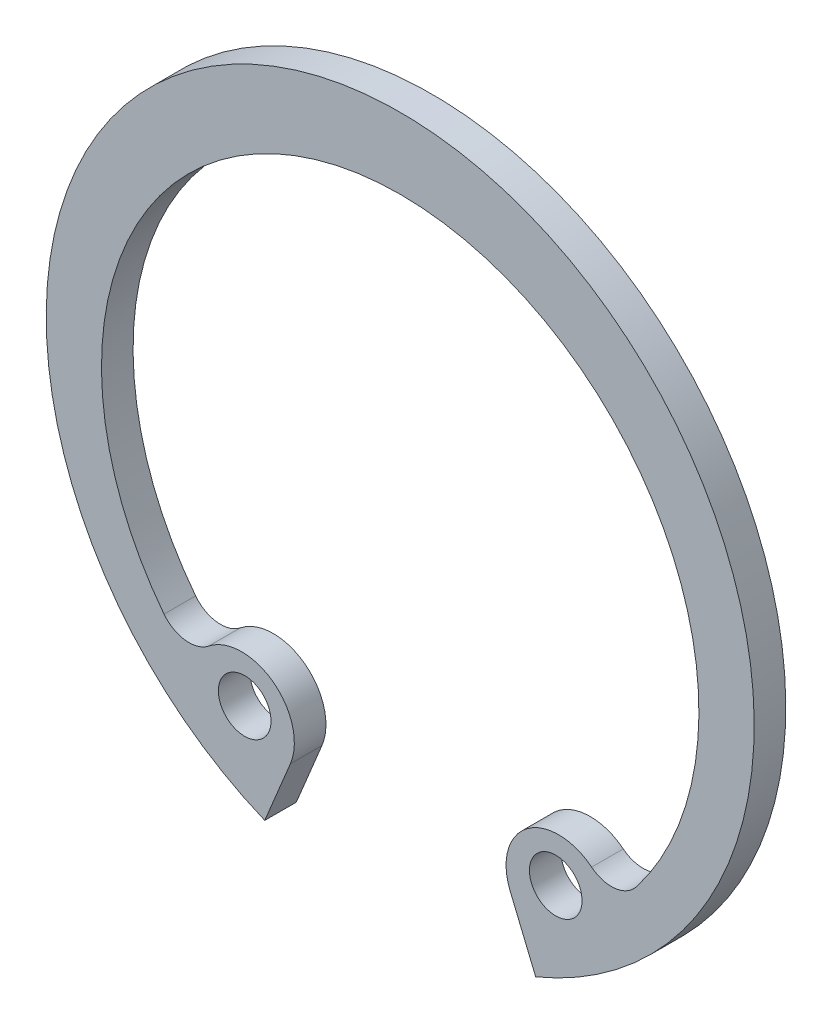
from build123d import *

# Parameters (mm, degrees)
SKETCH1_R          = 1
BASE_EXTRUDE_DEPTH = 1.2


with BuildPart() as part:
    # Sketch1 → Base-Extrude (new body)
    with BuildSketch(Plane.XY):
        with BuildLine():
            Line((-4.17437466, -10.077831919), (-5.147092165, -12.426179712))
            ThreePointArc((-5.147092165, -12.426179712), (0, 13.45), (5.147092165, -12.426179712))
            Line((5.147092165, -12.426179712), (4.17437466, -10.077831919))
            ThreePointArc((4.17437466, -10.077831919), (4.821639244, -7.712836035), (7.273294145, -7.752145343))
            ThreePointArc((7.273294145, -7.752145343), (8.165152835, -8.007621744), (8.972639508, -7.550844571))
            ThreePointArc((8.972639508, -7.550844571), (0, 10.75), (-8.972639508, -7.550844571))
            ThreePointArc((-8.972639508, -7.550844571), (-8.165152835, -8.007621744), (-7.273294145, -7.752145343))
            ThreePointArc((-7.273294145, -7.752145343), (-4.821639244, -7.712836035), (-4.17437466, -10.077831919))
        make_face()
        with Locations((-5.909254613, -9.03995077)):
            Circle(SKETCH1_R, mode=Mode.SUBTRACT)
        with Locations(Location((5.909254613, -9.03995077, 0), (0, 0, 180))):
            Circle(SKETCH1_R, mode=Mode.SUBTRACT)
    extrude(amount=BASE_EXTRUDE_DEPTH)


solid = part.part
